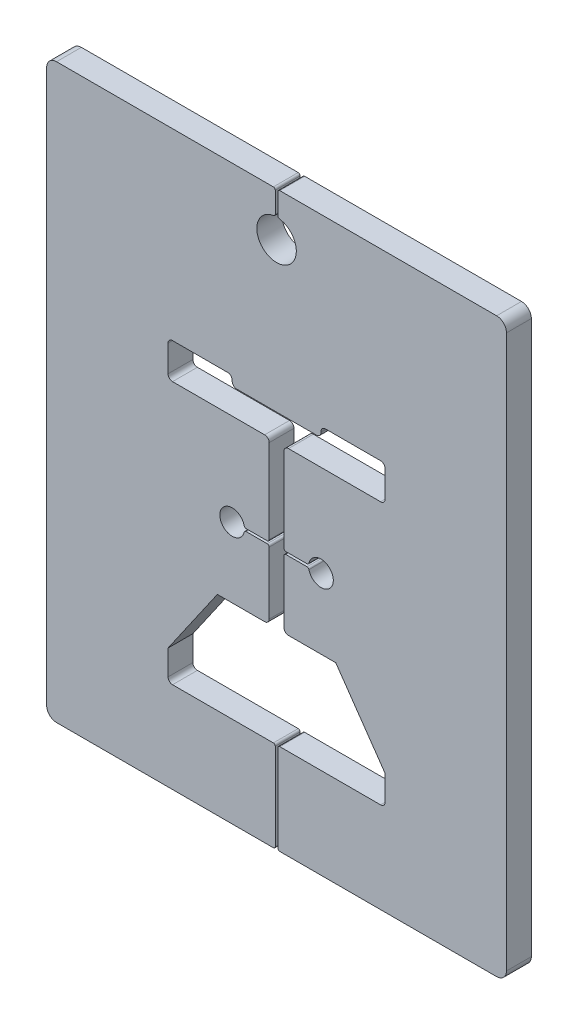
from build123d import *

# Parameters (mm, degrees)
BOSS_EXTRUDE1_DEPTH = 32


with BuildPart() as part:
    # Sketch1 → Boss-Extrude1 (new body)
    with BuildSketch(Plane.XY):
        with BuildLine():
            Line((-473.771437729, 649.485465586), (-194.711437729, 649.485465586))
            ThreePointArc((-194.711437729, 649.485465586), (-192.943670776, 648.753232539), (-192.211437729, 646.985465586))
            Line((-192.211437729, 646.985465586), (-192.211437729, 620.183304835))
            ThreePointArc((-192.211437729, 620.183304835), (-192.816753125, 618.552301999), (-194.33957393, 617.711116065))
            ThreePointArc((-194.33957393, 617.711116065), (-190.561437729, 567.193678161), (-186.783301529, 617.711116065))
            ThreePointArc((-186.783301529, 617.711116065), (-188.306122334, 618.552301999), (-188.911437729, 620.183304835))
            Line((-188.911437729, 620.183304835), (-188.911437729, 646.985465586))
            ThreePointArc((-188.911437729, 646.985465586), (-188.179204682, 648.753232539), (-186.411437729, 649.485465586))
            Line((-186.411437729, 649.485465586), (92.648562271, 649.485465586))
            ThreePointArc((92.648562271, 649.485465586), (101.628818392, 645.765721708), (105.348562271, 636.785465586))
            Line((105.348562271, 636.785465586), (105.348562271, -74.414534414))
            ThreePointArc((105.348562271, -74.414534414), (101.628818392, -83.394790535), (92.648562271, -87.114534414))
            Line((92.648562271, -87.114534414), (-186.411437729, -87.114534414))
            ThreePointArc((-186.411437729, -87.114534414), (-188.179204682, -86.382301366), (-188.911437729, -84.614534414))
            Line((-188.911437729, -84.614534414), (-188.911437729, 27.225465586))
            ThreePointArc((-188.911437729, 27.225465586), (-188.179204682, 28.993232539), (-186.411437729, 29.725465586))
            Line((-186.411437729, 29.725465586), (-56.661437729, 29.725465586))
            ThreePointArc((-56.661437729, 29.725465586), (-52.560218399, 31.424246256), (-50.861437729, 35.525465586))
            Line((-50.861437729, 35.525465586), (-50.861437729, 67.725465586))
            Line((-50.861437729, 67.725465586), (-114.361437729, 159.265465586))
            Line((-114.361437729, 159.265465586), (-175.236437729, 159.265465586))
            ThreePointArc((-175.236437729, 159.265465586), (-179.33765706, 160.964246256), (-181.036437729, 165.065465586))
            Line((-181.036437729, 165.065465586), (-181.036437729, 245.285465586))
            ThreePointArc((-181.036437729, 245.285465586), (-180.304204682, 247.053232539), (-178.536437729, 247.785465586))
            Line((-178.536437729, 247.785465586), (-151.311664683, 247.785465586))
            ThreePointArc((-151.311664683, 247.785465586), (-149.75628123, 247.242704027), (-148.876259656, 245.850091437))
            ThreePointArc((-148.876259656, 245.850091437), (-117.536437729, 249.435465586), (-148.876259656, 253.020839736))
            ThreePointArc((-148.876259656, 253.020839736), (-149.75628123, 251.628227146), (-151.311664683, 251.085465586))
            Line((-151.311664683, 251.085465586), (-178.536437729, 251.085465586))
            ThreePointArc((-178.536437729, 251.085465586), (-180.304204682, 251.817698634), (-181.036437729, 253.585465586))
            Line((-181.036437729, 253.585465586), (-181.036437729, 302.775884834))
            Line((-181.036437729, 302.775884834), (-181.036437729, 361.745465586))
            ThreePointArc((-181.036437729, 361.745465586), (-179.33765706, 365.846684917), (-175.236437729, 367.545465586))
            Line((-175.236437729, 367.545465586), (-56.656437729, 367.545465586))
            ThreePointArc((-56.656437729, 367.545465586), (-52.555218399, 369.244246256), (-50.856437729, 373.345465586))
            Line((-50.856437729, 373.345465586), (-50.856437729, 407.465465586))
            ThreePointArc((-50.856437729, 407.465465586), (-52.555218399, 411.566684917), (-56.656437729, 413.265465586))
            Line((-56.656437729, 413.265465586), (-127.611437729, 413.265465586))
            ThreePointArc((-127.611437729, 413.265465586), (-131.71265706, 411.566684917), (-133.411437729, 407.465465586))
            Line((-133.411437729, 407.465465586), (-133.411437729, 406.365465586))
            ThreePointArc((-133.411437729, 406.365465586), (-135.110218399, 402.264246256), (-139.211437729, 400.565465586))
            Line((-139.211437729, 400.565465586), (-241.911437729, 400.565465586))
            ThreePointArc((-241.911437729, 400.565465586), (-246.01265706, 402.264246256), (-247.711437729, 406.365465586))
            Line((-247.711437729, 406.365465586), (-247.711437729, 407.465465586))
            ThreePointArc((-247.711437729, 407.465465586), (-249.410218399, 411.566684917), (-253.511437729, 413.265465586))
            Line((-253.511437729, 413.265465586), (-324.466437729, 413.265465586))
            ThreePointArc((-324.466437729, 413.265465586), (-328.56765706, 411.566684917), (-330.266437729, 407.465465586))
            Line((-330.266437729, 407.465465586), (-330.266437729, 373.345465586))
            ThreePointArc((-330.266437729, 373.345465586), (-328.56765706, 369.244246256), (-324.466437729, 367.545465586))
            Line((-324.466437729, 367.545465586), (-205.886437729, 367.545465586))
            ThreePointArc((-205.886437729, 367.545465586), (-201.785218399, 365.846684917), (-200.086437729, 361.745465586))
            Line((-200.086437729, 361.745465586), (-200.086437729, 302.775884834))
            Line((-200.086437729, 302.775884834), (-200.086437729, 253.585465586))
            ThreePointArc((-200.086437729, 253.585465586), (-200.818670776, 251.817698634), (-202.586437729, 251.085465586))
            Line((-202.586437729, 251.085465586), (-229.811210776, 251.085465586))
            ThreePointArc((-229.811210776, 251.085465586), (-231.366594229, 251.628227146), (-232.246615803, 253.020839736))
            ThreePointArc((-232.246615803, 253.020839736), (-263.586437729, 249.435465586), (-232.246615803, 245.850091437))
            ThreePointArc((-232.246615803, 245.850091437), (-231.366594229, 247.242704027), (-229.811210776, 247.785465586))
            Line((-229.811210776, 247.785465586), (-202.586437729, 247.785465586))
            ThreePointArc((-202.586437729, 247.785465586), (-200.818670776, 247.053232539), (-200.086437729, 245.285465586))
            Line((-200.086437729, 245.285465586), (-200.086437729, 165.065465586))
            ThreePointArc((-200.086437729, 165.065465586), (-201.785218399, 160.964246256), (-205.886437729, 159.265465586))
            Line((-205.886437729, 159.265465586), (-266.761437729, 159.265465586))
            Line((-266.761437729, 159.265465586), (-330.261437729, 67.725465586))
            Line((-330.261437729, 67.725465586), (-330.261437729, 35.525465586))
            ThreePointArc((-330.261437729, 35.525465586), (-328.56265706, 31.424246256), (-324.461437729, 29.725465586))
            Line((-324.461437729, 29.725465586), (-194.711437729, 29.725465586))
            ThreePointArc((-194.711437729, 29.725465586), (-192.943670776, 28.993232539), (-192.211437729, 27.225465586))
            Line((-192.211437729, 27.225465586), (-192.211437729, -84.614534414))
            ThreePointArc((-192.211437729, -84.614534414), (-192.943670776, -86.382301366), (-194.711437729, -87.114534414))
            Line((-194.711437729, -87.114534414), (-473.771437729, -87.114534414))
            ThreePointArc((-473.771437729, -87.114534414), (-482.751693851, -83.394790535), (-486.471437729, -74.414534414))
            Line((-486.471437729, -74.414534414), (-486.471437729, 636.785465586))
            ThreePointArc((-486.471437729, 636.785465586), (-482.751693851, 645.765721708), (-473.771437729, 649.485465586))
        make_face()
    extrude(amount=BOSS_EXTRUDE1_DEPTH)


solid = part.part
